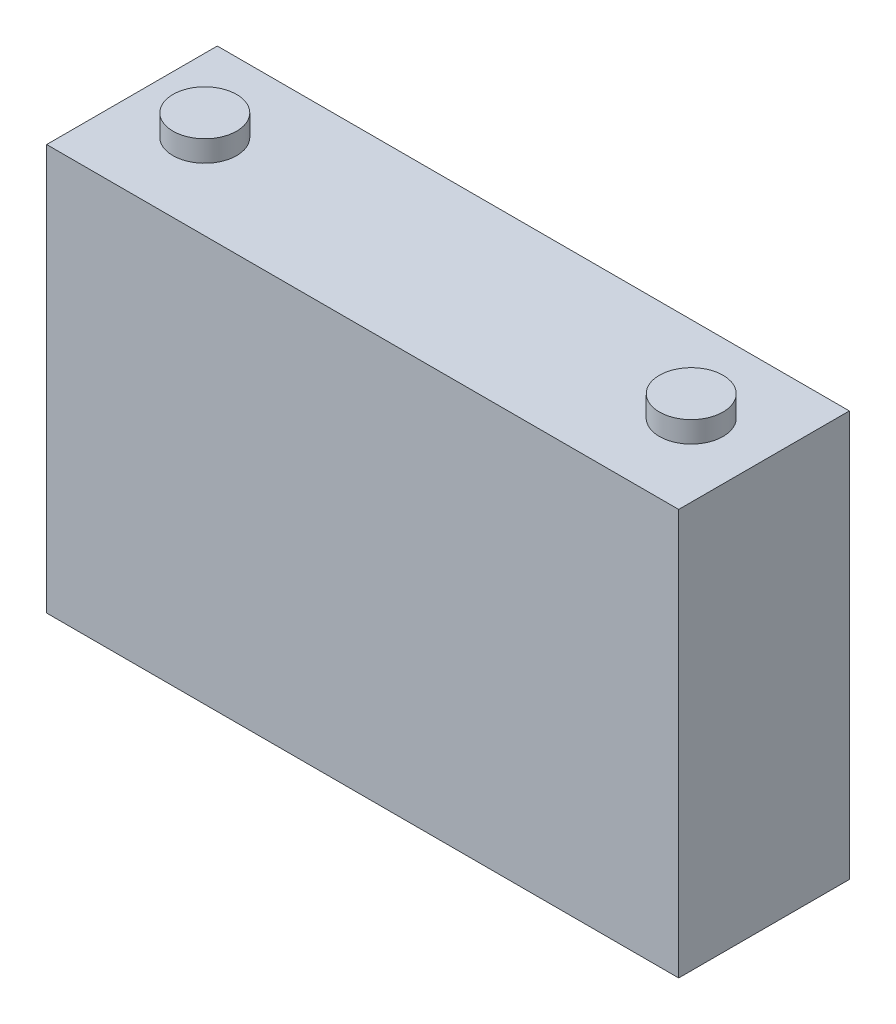
from build123d import *

# Parameters (mm, degrees)
SKETCH_1_W      = 148.9
SKETCH_1_H      = 40.2
EXTRUDE_1_DEPTH = 95.6
SKETCH_2_R      = 7.5
EXTRUDE_2_DEPTH = 5


with BuildPart() as part:
    # 草图1 → 凸台-拉伸1 (new body)
    with BuildSketch(Plane(origin=(0, 0, 0), x_dir=(1, 0, 0), z_dir=(0, 1, 0))):
        Rectangle(SKETCH_1_W, SKETCH_1_H)
    extrude(amount=EXTRUDE_1_DEPTH)

    # 草图2 → 凸台-拉伸2 (add)
    with BuildSketch(Plane(origin=(0, 95.6, 0), x_dir=(1, 0, 0), z_dir=(0, 1, 0))):
        with Locations(Location((57.3, 0, 0), (0, 0, 270))):
            Circle(SKETCH_2_R)
        with Locations(Location((-57.3, 0, 0), (0, 0, 270))):
            Circle(SKETCH_2_R)
    extrude(amount=EXTRUDE_2_DEPTH)


solid = part.part
